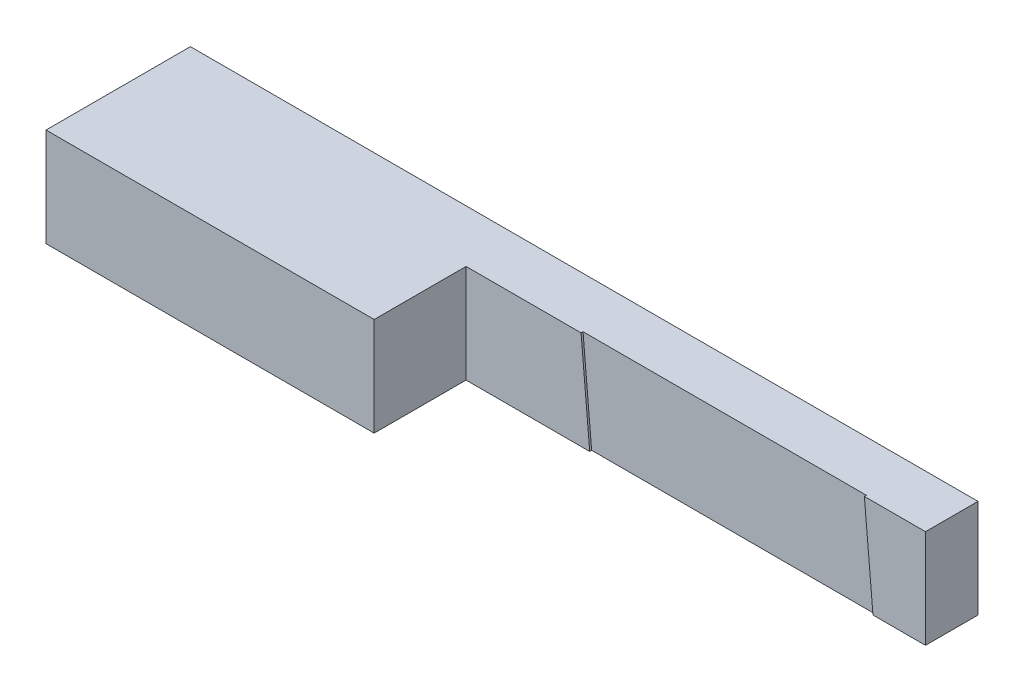
from build123d import *

# Parameters (mm, degrees)
SKETCH_1_W          = 120
SKETCH_1_H          = 15
EXTRUDE_1_DEPTH     = 8
CUT_EXTRUDE_1_DEPTH = 0.3
SKETCH_6_W          = 50
SKETCH_6_H          = 14
EXTRUDE_2_DEPTH     = 15


with BuildPart() as part:
    # 草图1 → 凸台-拉伸1 (new body)
    with BuildSketch(Plane.XY):
        Rectangle(SKETCH_1_W, SKETCH_1_H)
    extrude(amount=EXTRUDE_1_DEPTH)

    # 草图2 → 切除-拉伸1 (cut)
    with BuildSketch(Plane.XY.offset(8)):
        Polygon((50.687670047, 7.5), (52, -7.5), (8.835746986, -7.5), (7.523417033, 7.5), align=None)
    extrude(amount=-CUT_EXTRUDE_1_DEPTH, mode=Mode.SUBTRACT)

    # 草图6 → 凸台-拉伸2 (add)
    with BuildSketch(Plane.XZ.offset(7.5)):
        with Locations((-35, 15)):
            Rectangle(SKETCH_6_W, SKETCH_6_H)
    extrude(amount=-EXTRUDE_2_DEPTH)


solid = part.part
